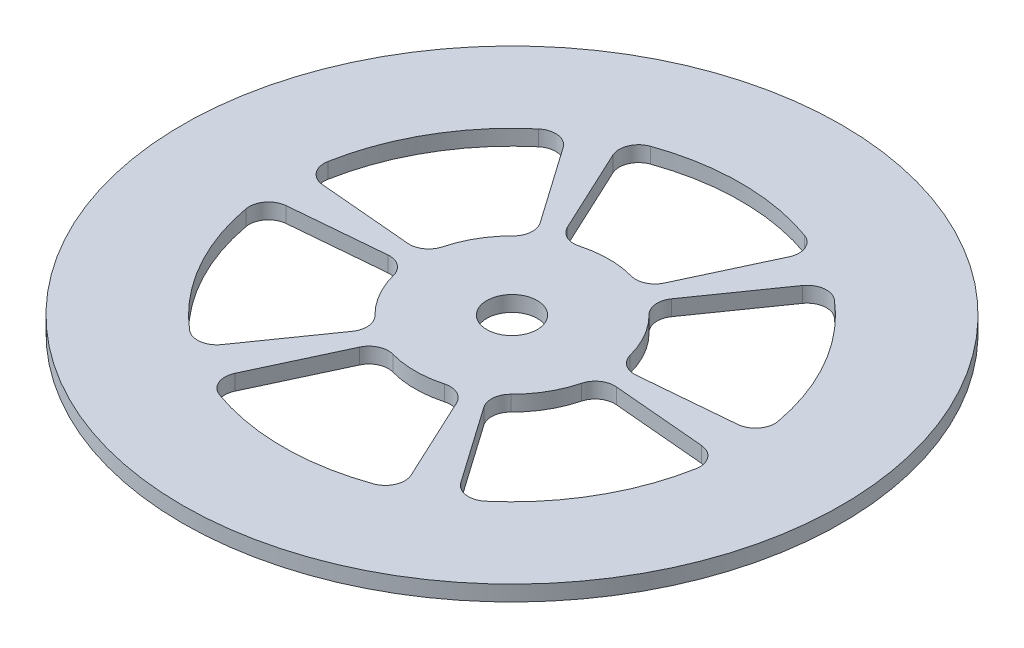
from build123d import *

# Parameters (mm, degrees)
SKETCH1_R           = 85
SKETCH1_R_2         = 6.5
BOSS_EXTRUDE1_DEPTH = 4
CUT_EXTRUDE1_DEPTH  = 10
FILLET1_R           = 5


with BuildPart() as part:
    # Sketch1 → Boss-Extrude1 (new body)
    with BuildSketch(Plane(origin=(0, 0, 0), x_dir=(1, 0, 0), z_dir=(0, 1, 0))):
        with Locations(Location((0, 0, 0), (0, 0, 270))):
            Circle(SKETCH1_R)
        with Locations(Location((0, 0, 0), (0, 0, 270))):
            Circle(SKETCH1_R_2, mode=Mode.SUBTRACT)
    extrude(amount=BOSS_EXTRUDE1_DEPTH)

    # Sketch2 → Cut-Extrude1 (cut)
    with BuildSketch(Plane(origin=(0, 4, 0), x_dir=(1, 0, 0), z_dir=(0, 1, 0))):
        with BuildLine():
            Line((10.565456544, 22.657694676), (24.934477443, 53.472159435))
            ThreePointArc((24.934477443, 53.472159435), (0, 59), (-24.934477443, 53.472159435))
            Line((-24.934477443, 53.472159435), (-10.565456544, 22.657694676))
            ThreePointArc((-10.565456544, 22.657694676), (0, 25), (10.565456544, 22.657694676))
        make_face()
        with BuildLine():
            Line((14.339410909, 20.478801107), (33.841009745, 48.329970613))
            ThreePointArc((33.841009745, 48.329970613), (51.095498823, 29.5), (58.775487187, 5.142188822))
            Line((58.775487187, 5.142188822), (24.904867452, 2.178893569))
            ThreePointArc((24.904867452, 2.178893569), (21.650635095, 12.5), (14.339410909, 20.478801107))
        make_face()
        with BuildLine():
            Line((24.904867452, -2.178893569), (58.775487187, -5.142188822))
            ThreePointArc((58.775487187, -5.142188822), (51.095498823, -29.5), (33.841009745, -48.329970613))
            Line((33.841009745, -48.329970613), (14.339410909, -20.478801107))
            ThreePointArc((14.339410909, -20.478801107), (21.650635095, -12.5), (24.904867452, -2.178893569))
        make_face()
        with BuildLine():
            Line((10.565456544, -22.657694676), (24.934477443, -53.472159435))
            ThreePointArc((24.934477443, -53.472159435), (0, -59), (-24.934477443, -53.472159435))
            Line((-24.934477443, -53.472159435), (-10.565456544, -22.657694676))
            ThreePointArc((-10.565456544, -22.657694676), (0, -25), (10.565456544, -22.657694676))
        make_face()
        with BuildLine():
            Line((-14.339410909, -20.478801107), (-33.841009745, -48.329970613))
            ThreePointArc((-33.841009745, -48.329970613), (-51.095498823, -29.5), (-58.775487187, -5.142188822))
            Line((-58.775487187, -5.142188822), (-24.904867452, -2.178893569))
            ThreePointArc((-24.904867452, -2.178893569), (-21.650635095, -12.5), (-14.339410909, -20.478801107))
        make_face()
        with BuildLine():
            Line((-24.904867452, 2.178893569), (-58.775487187, 5.142188822))
            ThreePointArc((-58.775487187, 5.142188822), (-51.095498823, 29.5), (-33.841009745, 48.329970613))
            Line((-33.841009745, 48.329970613), (-14.339410909, 20.478801107))
            ThreePointArc((-14.339410909, 20.478801107), (-21.650635095, 12.5), (-24.904867452, 2.178893569))
        make_face()
    extrude(amount=-CUT_EXTRUDE1_DEPTH, mode=Mode.SUBTRACT)

    # Fillet1
    fillet1_edges = [part.edges().sort_by_distance(p)[0] for p in [
        (-10.565456544, 2, 22.657694676),
        (10.565456544, 2, 22.657694676),
        (24.934477443, 2, 53.472159435),
        (-24.934477443, 2, 53.472159435),
        (-24.904867452, 2, 2.178893569),
        (-14.339410909, 2, 20.478801107),
        (-33.841009745, 2, 48.329970613),
        (-58.775487187, 2, 5.142188822),
        (14.339410909, 2, 20.478801107),
        (24.904867452, 2, 2.178893569),
        (58.775487187, 2, 5.142188822),
        (33.841009745, 2, 48.329970613),
        (24.904867452, 2, -2.178893569),
        (14.339410909, 2, -20.478801107),
        (33.841009745, 2, -48.329970613),
        (58.775487187, 2, -5.142188822),
        (-14.339410909, 2, -20.478801107),
        (-24.904867452, 2, -2.178893569),
        (-58.775487187, 2, -5.142188822),
        (-33.841009745, 2, -48.329970613),
        (10.565456544, 2, -22.657694676),
        (-10.565456544, 2, -22.657694676),
        (-24.934477443, 2, -53.472159435),
        (24.934477443, 2, -53.472159435),
    ]]
    fillet(fillet1_edges, radius=FILLET1_R)


solid = part.part
